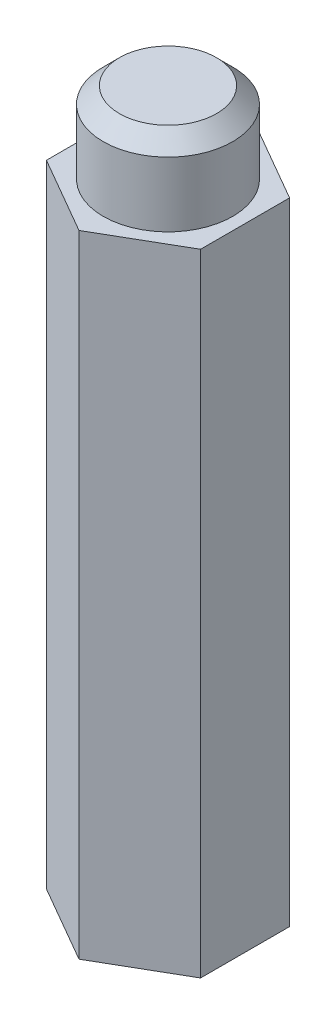
SolidWorks part; units mm, degrees
ref_plane "Front Plane" through (0, 0, 0) normal (0, 0, 1) x (1, 0, 0)
ref_plane "Top Plane" through (0, 0, 0) normal (0, 1, 0) x (1, 0, 0)
ref_plane "Right Plane" through (0, 0, 0) normal (1, 0, 0) x (0, 0, -1)
sketch "Sketch1" plane through (0, 0, 0) normal (0, 1, 0) x (1, 0, 0)
  line L1 (0, 5.5) -> (-4.7631, 2.75)
  line L2 (-4.7631, 2.75) -> (-4.7631, -2.75)
  line L3 (-4.7631, -2.75) -> (0, -5.5)
  line L4 (0, -5.5) -> (4.7631, -2.75)
  line L5 (4.7631, -2.75) -> (4.7631, 2.75)
  line L6 (4.7631, 2.75) -> (0, 5.5)
  circle A0 centre (0, 0) radius 4.7631 construction
  dimension "D1" = 11
extrude "Boss-Extrude1" add sketch "Sketch1" along normal mid plane 39
sketch "Sketch3" plane through (0, 19.5, 0) normal (0, 1, 0) x (1, 0, 0)
  circle A0 centre (0, 0) radius 4
  dimension "D1" = 8
extrude "Boss-Extrude2" add sketch "Sketch3" along normal blind 5
chamfer "Chamfer1" distance 1 angle 45 1 edges at (0, 24.5, 4)
hole_wizard "M6x1.0 Tapped Hole2" positions "3DSketch1" profile "Sketch6" tap size "M6x1.0" standard "ANSI Metric"
sketch3d "3DSketch1"
  point P0 (0, 0, 0)
  point P4 (0, -19.5, 0)
sketch "Sketch6" plane through (0, -19.5, 0) normal (1, 0, 0) x (0, 0, -1)
  line L0 (0, 0) -> (0, 9.5022)
  line L1 (0, 9.5022) -> (2.5, 8)
  line L2 (2.5, 8) -> (2.5, 0)
  line L5 (2.5, 0) -> (0, 0)
  line L10 (0, 9.5022) -> (-2.5, 8) construction
  line L11 (0, -6.35) -> (0, 107.95) construction
  dimension "Tap Drill Dia." = 5
  dimension "Tap Drill Depth" = 8
  dimension "Drill Angle" = 118
cosmetic thread "Hole Thread2" parameters "D1"=4, "D2"=6
cosmetic thread "Hole Thread3" parameters "D1"=4, "D2"=6
